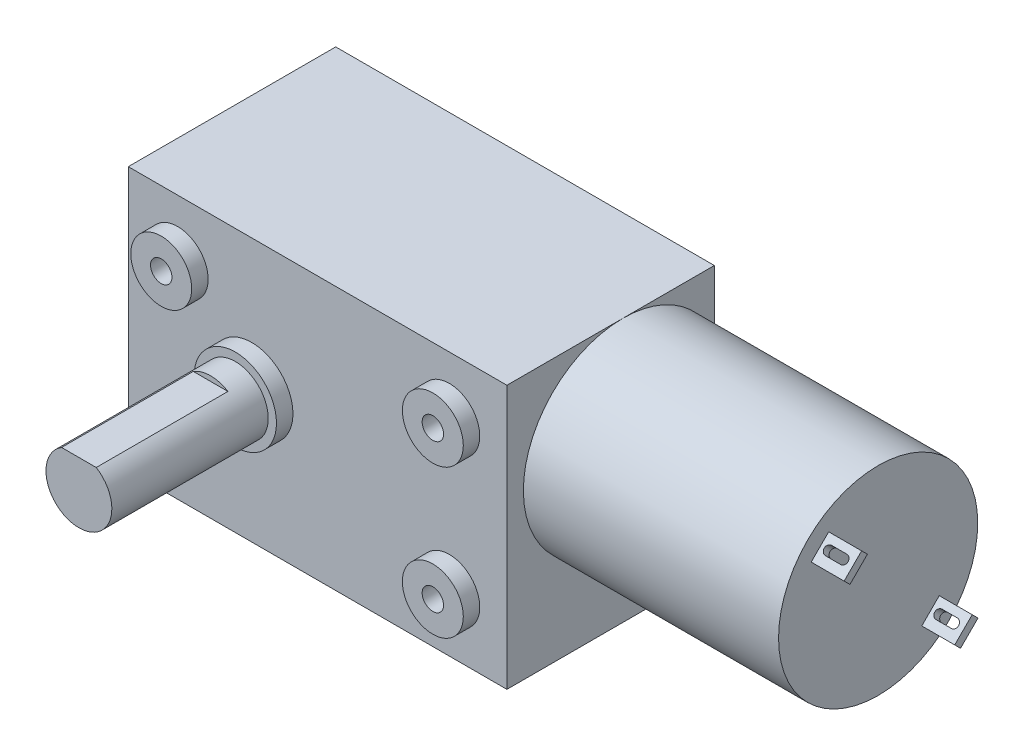
SolidWorks part; units mm, degrees
ref_plane "前视基准面" through (0, 0, 0) normal (0, 0, 1) x (1, 0, 0)
ref_plane "上视基准面" through (0, 0, 0) normal (0, 1, 0) x (1, 0, 0)
ref_plane "右视基准面" through (0, 0, 0) normal (1, 0, 0) x (0, 0, -1)
sketch "草图1" plane through (0, 0, 0) normal (0, 0, 1) x (1, 0, 0)
  line L1 (0, 0) -> (46, 0)
  line L2 (0, 0) -> (0, 32)
  line L3 (0, 32) -> (46, 32)
  line L4 (46, 0) -> (46, 32)
  dimension "D1" = 32
  dimension "D2" = 46
extrude "凸台-拉伸1" add sketch "草图1" along normal blind 25.2
sketch "草图2" plane through (0, 0, 25.2) normal (0, 0, 1) x (1, 0, 0)
  line L0 (46, 32) -> (0, 32) construction
  line L3 (0, 32) -> (0, 0) construction
  line L4 (6, 25) -> (39, 25) construction
  line L5 (6, 25) -> (6, 7) construction
  line L6 (6, 7) -> (39, 7) construction
  line L7 (39, 25) -> (39, 7) construction
  circle A0 centre (6, 25) radius 3.7
  circle A1 centre (6, 7) radius 3.7
  circle A2 centre (39, 7) radius 3.7
  circle A3 centre (39, 25) radius 3.7
  circle A4 centre (15, 16) radius 5
  dimension "D5" = 7.4
  dimension "D6" = 7.4
  dimension "D7" = 7.4
  dimension "D8" = 7.4
  dimension "D9" = 15
  dimension "D10" = 16
  dimension "D11" = 10
  dimension "D1" = 18
  dimension "D2" = 7
  dimension "D3" = 33
  dimension "D4" = 6
extrude "凸台-拉伸2" add sketch "草图2" along normal blind 2
sketch "草图3" plane through (0, 0, 27.2) normal (0, 0, 1) x (1, 0, 0)
  circle A0 centre (6, 7) radius 1.3
  circle A1 centre (6, 25) radius 1.3
  circle A2 centre (39, 25) radius 1.3
  circle A3 centre (39, 7) radius 1.3
  dimension "D1" = 2.6
  dimension "D2" = 2.6
  dimension "D3" = 2.6
  dimension "D4" = 2.6
extrude "切除-拉伸1" cut sketch "草图3" against normal blind 10
cosmetic thread "装饰螺纹线1" parameters "D2"=3
cosmetic thread "装饰螺纹线2" parameters "D2"=3
cosmetic thread "装饰螺纹线3" parameters "D2"=3
cosmetic thread "装饰螺纹线4" parameters "D2"=3
sketch "草图4" plane through (0, 0, 27.2) normal (0, 0, 1) x (1, 0, 0)
  circle A0 centre (15, 16) radius 4
extrude "凸台-拉伸3" add sketch "草图4" along normal blind 19
sketch "草图5" plane through (0, 0, 46.2) normal (0, 0, 1) x (1, 0, 0)
  line L1 (17.1071, 19.4) -> (12.8929, 19.4)
  arc A2 (17.1071, 19.4) -> (12.8929, 19.4) centre (15, 16) ccw
  dimension "D1" = 4
  dimension "D2" = 3.4
extrude "切除-拉伸2" cut sketch "草图5" against normal blind 16
sketch "草图6" plane through (46, 0, 0) normal (1, 0, 0) x (0, 0, -1)
  circle A0 centre (-11.1, 19.9) radius 12.1
extrude "凸台-拉伸4" add sketch "草图6" along normal blind 31
sketch "草图7" plane through (77, 0, 0) normal (1, 0, 0) x (0, 0, -1)
  line L1 (-19.2317, 25.9104) -> (-17.1104, 28.0317)
  line L2 (-19.2317, 25.9104) -> (-18.5246, 25.2033)
  line L3 (-18.5246, 25.2033) -> (-16.4033, 27.3246)
  line L4 (-17.1104, 28.0317) -> (-16.4033, 27.3246)
  line L5 (-5.7967, 12.4754) -> (-3.6754, 14.5967)
  line L6 (-5.7967, 12.4754) -> (-5.0896, 11.7683)
  line L7 (-5.0896, 11.7683) -> (-2.9683, 13.8896)
  line L8 (-3.6754, 14.5967) -> (-2.9683, 13.8896)
  circle A0 centre (-11.1, 19.9) radius 12.1 construction
  dimension "D1" = 0
  dimension "D2" = 1
  dimension "D3" = 1
  dimension "D4" = 18
  dimension "D5" = 9
  dimension "D6" = 3
  dimension "D7" = 1.5
  dimension "D8" = 3
extrude "凸台-拉伸5" add sketch "草图7" along normal blind 4
sketch "草图8" plane through (0, 22.5711, 22.5711) normal (0, 0.7071, 0.7071) x (1, 0, 0)
  line L0 (77.9693, 6.3228) -> (79.8219, 6.3228) construction
  line L1 (77.9693, 6.8423) -> (79.8219, 6.8423)
  line L2 (77.9693, 5.8034) -> (79.8219, 5.8034)
  arc A0 (77.9693, 6.8423) -> (77.9693, 5.8034) centre (77.9693, 6.3228) ccw
  arc A1 (79.8219, 5.8034) -> (79.8219, 6.8423) centre (79.8219, 6.3228) ccw
  point P2 (78.8956, 6.3228)
extrude "切除-拉伸3" cut sketch "草图8" against normal through all
